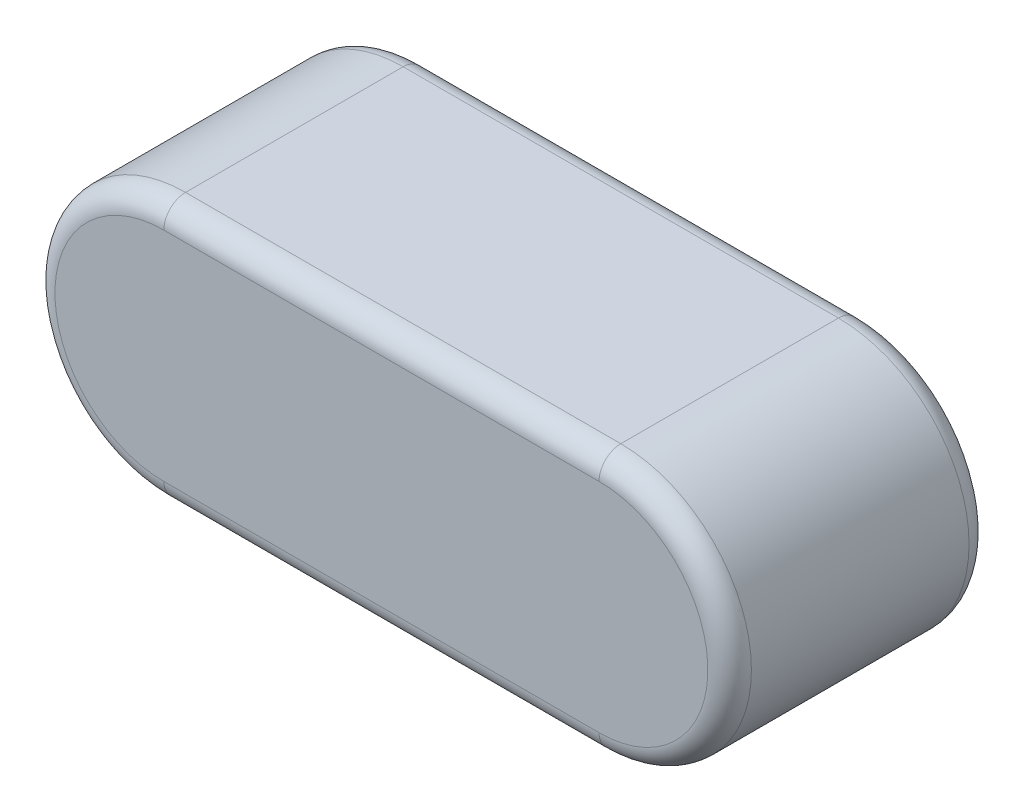
SolidWorks part; units mm, degrees
ref_plane "Plane1" through (0, 0, 0) normal (0, 0, 1) x (1, 0, 0)
ref_plane "Plane2" through (0, 0, 0) normal (0, 1, 0) x (1, 0, 0)
ref_plane "Plane3" through (0, 0, 0) normal (1, 0, 0) x (0, 0, -1)
sketch "Dimension Sketch" plane through (0, 0, 0) normal (0, 0, 1) x (1, 0, 0)
  line L0 (-4, 0) -> (4, 0) construction
  point P3 (-3, 0)
  point P4 (-0.25, 0)
  point P5 (0, 0)
  point P8 (-3, 0)
  point P11 (0, 0)
sketch "Sketch1" plane through (0, 0, 0) normal (0, 0, 1) x (1, 0, 0)
  line L0 (-28.0599, 0) -> (30.562, 0) construction
  line L1 (-2.5, 1.5) -> (2.5, 1.5)
  line L2 (-2.5, -1.5) -> (2.5, -1.5)
  line L3 (0, 2.9108) -> (0, -2.1805) construction
  arc A0 (-2.5, 1.5) -> (-2.5, -1.5) centre (-2.5, 0) ccw
  arc A1 (2.5, 1.5) -> (2.5, -1.5) centre (2.5, 0) cw
extrude "Base-Extrude" add sketch "Sketch1" along normal blind 3
fillet "Fillet1" radius 0.25 8 edges at (4, 0, 3) (0, 1.5, 3) (-4, 0, 3) (0, 1.5, 0) (4, 0, 0) (0, -1.5, 0) (-4, 0, 0) (0, -1.5, 3)
equation "\"D3@Sketch1\" = \"L@Dimension Sketch\""
equation "\"D1@Sketch1\" = \"b@Dimension Sketch\" / 2"
equation "\"D1@Fillet1\" = \"r@Dimension Sketch\""
equation "\"D1@Base-Extrude\" = \"h@Dimension Sketch\""
